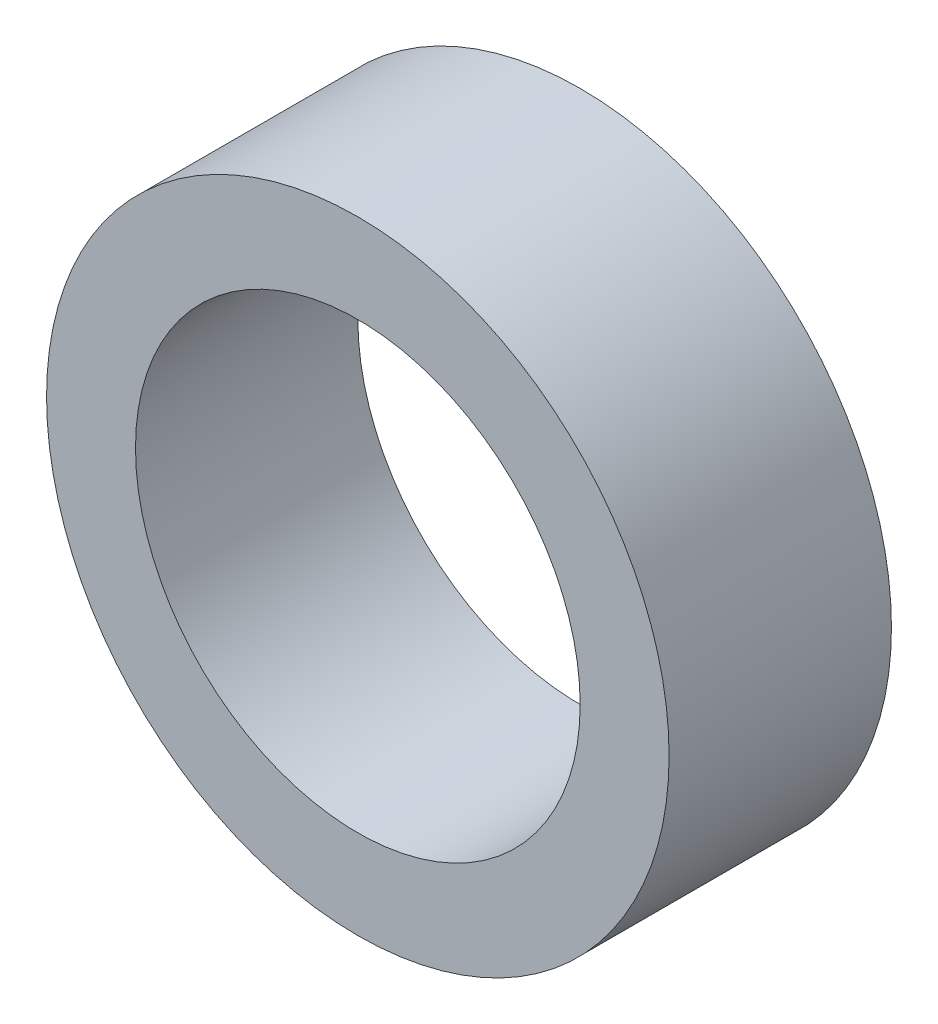
SolidWorks part; units mm, degrees
ref_plane "前视基准面" through (0, 0, 0) normal (0, 0, 1) x (1, 0, 0)
ref_plane "上视基准面" through (0, 0, 0) normal (0, 1, 0) x (1, 0, 0)
ref_plane "右视基准面" through (0, 0, 0) normal (1, 0, 0) x (0, 0, -1)
sketch "草图2" plane through (0, 0, 0) normal (0, 0, 1) x (1, 0, 0)
  circle A0 centre (0, 0) radius 10
  circle A1 centre (0, 0) radius 14
extrude "凸台-拉伸1" add sketch "草图2" along normal blind 10
